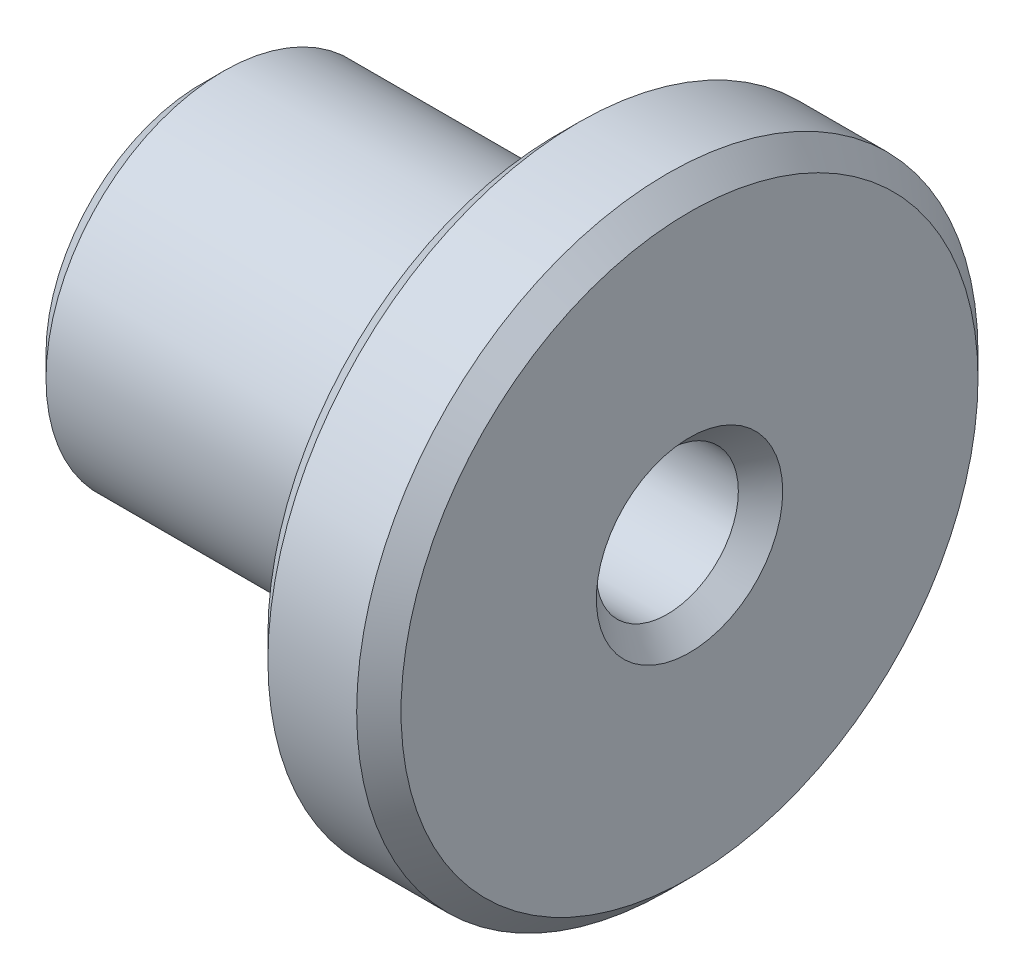
SolidWorks part; units mm, degrees
material "45"
ref_plane "Front Plane" through (0, 0, 0) normal (0, 0, 1) x (1, 0, 0)
ref_plane "Top Plane" through (0, 0, 0) normal (0, 1, 0) x (1, 0, 0)
ref_plane "Right Plane" through (0, 0, 0) normal (1, 0, 0) x (0, 0, -1)
sketch "Sketch1" plane through (0, 0, 0) normal (0, 0, 1) x (1, 0, 0)
  line L1 (6.5, 30.0426) -> (14.5, 30.0426)
  line L2 (14.5, 30.0426) -> (14.5, 33.0426)
  line L3 (14.5, 32.0426) -> (14.5, 21.0426) construction
  line L4 (14.5, 33.0426) -> (17.5, 33.0426)
  line L5 (17.5, 33.0426) -> (17.5, 27.6426)
  line L6 (17.5, 26.0426) -> (6.5, 26.0426) construction
  line L7 (6.5, 32.0426) -> (6.5, 21.0426) construction
  line L8 (17.5, 27.6426) -> (6.5, 27.6426)
  line L9 (6.5, 30.0426) -> (6.5, 27.6426)
  dimension "D1" = 3
  dimension "D2" = 3
  dimension "D3" = 7
  dimension "D4" = 2.4
revolve "Revolve1" add sketch "Sketch1" angle 360 about L6
chamfer "Chamfer1" distance 0.5 angle 45 4 edges at (14.5, 26.0426, -7) (17.5, 26.0426, -7) (6.5, 26.0426, -4) (17.5, 26.0426, -1.6)
